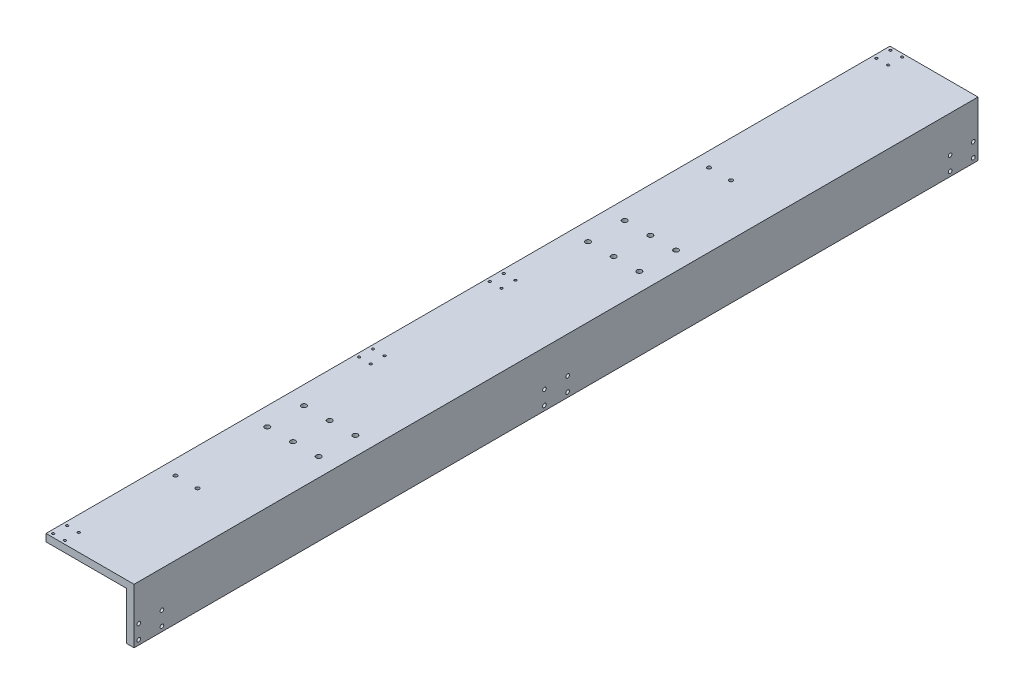
from build123d import *

# Parameters (mm, degrees)
EXTRUDE_1_DEPTH    = 575
HOLE_WIZARD_M4_1_D = 3.3
HOLE_WIZARD_M6_1_D = 5
HOLE_WIZARD_M8_1_D = 6.8
HOLE_WIZARD_M6_2_D = 5


with BuildPart() as part:
    # 草图1 → 凸台-拉伸1 (new, symmetric)
    with BuildSketch(Plane.XY):
        Polygon((0, 0), (120, 0), (120, -75), (110, -75), (110, -10), (0, -10), align=None)
    extrude(amount=EXTRUDE_1_DEPTH, both=True)

    # M4 螺纹孔1 (through all)
    with Locations(Plane(origin=(0, 0, 0), x_dir=(1, 0, 0), z_dir=(0, 1, 0))):
        with Locations((5.2, 43.6), (21.1, 43.6), (5.2, 24.6), (21.1, 24.6), (5.2, -134.6), (21.1, -134.6), (5.2, -153.6), (21.1, -153.6), (5.2, -551.4), (21.1, -551.4), (5.2, -570.4), (21.1, -570.4), (5.2, 570.4), (21.1, 570.4), (21.1, 551.4), (5.2, 551.4)):
            Hole(HOLE_WIZARD_M4_1_D / 2)

    # M6 螺纹孔1 (through all)
    with Locations(Plane(origin=(0, 0, 0), x_dir=(1, 0, 0), z_dir=(0, 1, 0))):
        with Locations((20, 308.5), (50, 308.5), (20, -418.5), (50, -418.5)):
            Hole(HOLE_WIZARD_M6_1_D / 2)

    # M8 螺纹孔1 (through all)
    with Locations(Plane(origin=(0, 0, 0), x_dir=(1, 0, 0), z_dir=(0, 1, 0))):
        with Locations((25, 188.5), (60, 188.5), (95, 188.5), (95, 138.5), (60, 138.5), (25, 138.5), (25, -248.5), (60, -248.5), (95, -248.5), (95, -298.5), (60, -298.5), (25, -298.5)):
            Hole(HOLE_WIZARD_M8_1_D / 2)

    # M6 螺纹孔2 (through all)
    with Locations(Plane(origin=(120, 0, 0), x_dir=(0, 0, -1), z_dir=(1, 0, 0))):
        with Locations((-568.6, -49.6), (-537, -49.6), (-537, -68.6), (-568.6, -68.6), (-15.8, -49.6), (15.8, -49.6), (15.8, -68.6), (-15.8, -68.6), (537, -49.6), (568.6, -49.6), (568.6, -68.6), (537, -68.6)):
            Hole(HOLE_WIZARD_M6_2_D / 2)


solid = part.part
